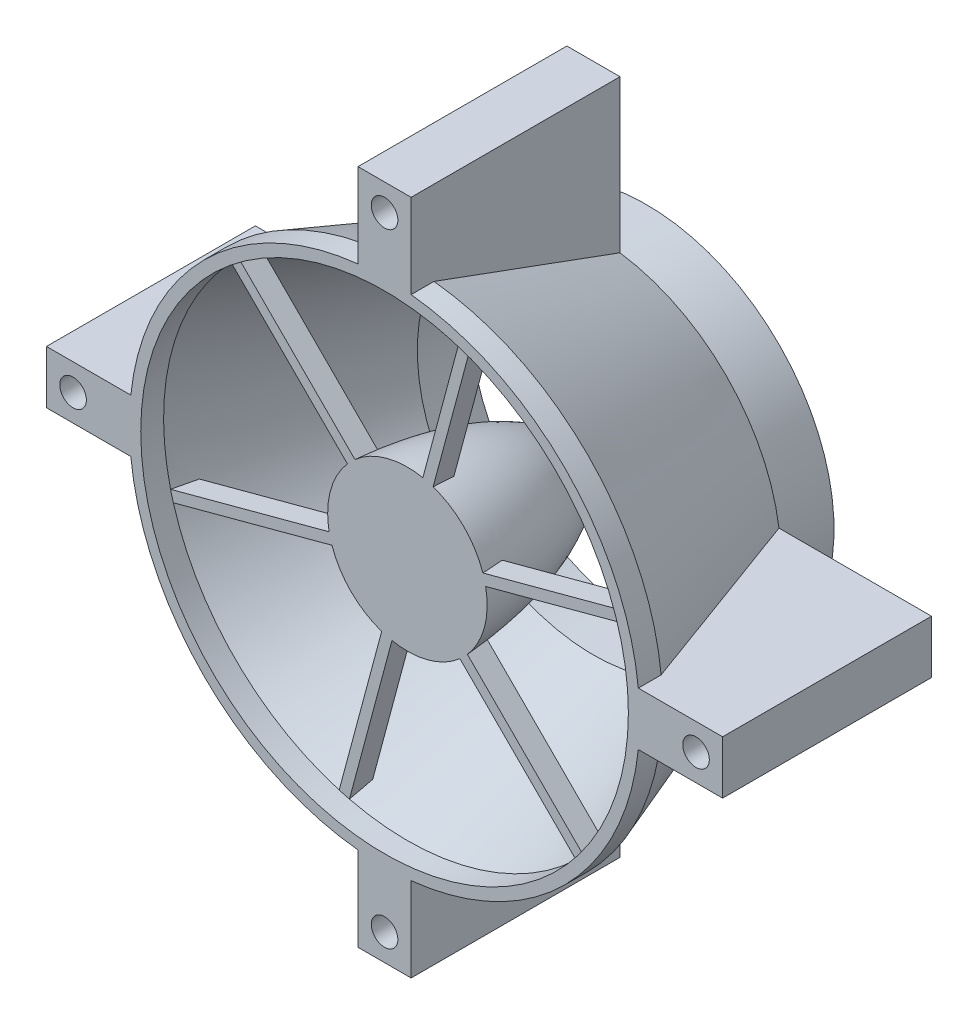
from build123d import *

# Parameters (mm, degrees)
SHELL2_T             = -2
BOSS_EXTRUDE10_REACH = 128.426
SKETCH20_W           = 10
SKETCH20_H           = 35
SKETCH21_R           = 2.5
CUT_EXTRUDE3_DEPTH   = 88.028501079
CIRPATTERN3_COUNT    = 4
SKETCH22_R           = 35.261041801
SKETCH22_R_2         = 33.132686256
BOSS_EXTRUDE11_DEPTH = 10
BOSS_EXTRUDE12_START = -5.388079
SKETCH24_W           = 4
SKETCH24_H           = 2
BOSS_EXTRUDE12_DEPTH = 31.259724
CIRPATTERN4_COUNT    = 6
SKETCH25_R           = 45.871644455
BOSS_EXTRUDE13_DEPTH = 4.3
SKETCH26_R           = 2.5
CUT_EXTRUDE4_DEPTH   = 103.569049913
SKETCH27_R           = 2.5
CUT_EXTRUDE5_DEPTH   = 103.569049913
SKETCH28_R           = 2.5
CUT_EXTRUDE6_DEPTH   = 103.569049913


with BuildPart() as part:
    # Sketch18 → Revolve1 (revolve)
    with BuildSketch(Plane(origin=(0, 0, 0), x_dir=(1, 0, 0), z_dir=(0, 1, 0)), mode=Mode.PRIVATE) as revolve1_sk:
        Polygon((0, 0), (-48, 0), (-35.261041801, 35), (0, 35), align=None)
    revolve(revolve1_sk.sketch.rotate(Axis((0, 0, 0), (0, 0, -1)), 180), axis=Axis((0, 0, 0), (0, 0, -1)))

    # Shell2
    shell2_openings = [part.faces().sort_by_distance(p)[0] for p in [
        (0, 0, -35),
        (0, 0, 0),
    ]]
    offset(amount=SHELL2_T, openings=shell2_openings, kind=Kind.INTERSECTION)

    # Sketch20 → Boss-Extrude10 (add, up to next)
    with BuildSketch(Plane(origin=(0, 63.6, 0), x_dir=(1, 0, 0), z_dir=(0, 1, 0)), mode=Mode.PRIVATE) as boss_extrude10_sk1:
        with Locations((0, 17.5)):
            Rectangle(SKETCH20_W, SKETCH20_H)
    boss_extrude10_tool1 = extrude(boss_extrude10_sk1.sketch, amount=-BOSS_EXTRUDE10_REACH, mode=Mode.PRIVATE) - part.part
    boss_extrude10 = boss_extrude10_tool1.solids().sort_by_distance((0, 63.6, -17.5))[0]
    add(boss_extrude10)

    # Sketch21 → Cut-Extrude3 (cut, through all)
    with BuildSketch(Plane(origin=(0, 0, -35), x_dir=(-1, 0, 0), z_dir=(0, 0, -1))):
        with Locations((0, 58.6)):
            Circle(SKETCH21_R)
    cut_extrude3 = extrude(amount=-CUT_EXTRUDE3_DEPTH, mode=Mode.SUBTRACT)

    # CirPattern3: Boss-Extrude10, Cut-Extrude3 ×4 about axis
    cirpattern3_axis = Axis((0, 0, 0), (0, 0, 1))
    add([boss_extrude10.rotate(cirpattern3_axis, i * 360 / CIRPATTERN3_COUNT) for i in range(1, CIRPATTERN3_COUNT)])
    add([cut_extrude3.rotate(cirpattern3_axis, i * 360 / CIRPATTERN3_COUNT) for i in range(1, CIRPATTERN3_COUNT)], mode=Mode.SUBTRACT)

    # Sketch22 → Boss-Extrude11 (add)
    with BuildSketch(Plane(origin=(0, 0, -35), x_dir=(-1, 0, 0), z_dir=(0, 0, -1))):
        with Locations(Location((0, 0, 0), (0, 0, 171.848007917))):
            Circle(SKETCH22_R)
        with Locations(Location((0, 0, 0), (0, 0, 180))):
            Circle(SKETCH22_R_2, mode=Mode.SUBTRACT)
    extrude(amount=BOSS_EXTRUDE11_DEPTH)



with BuildPart() as body_2:
    # Sketch23 → Revolve2 (revolve)
    with BuildSketch(Plane(origin=(0, 0, 0), x_dir=(1, 0, 0), z_dir=(0, 1, 0))):
        with BuildLine():
            Line((0, 0), (-15, 0))
            add(Edge.make_bspline(
                [(-15, 0), (-14.134412254, 12.425116283), (-11.061625239, 27.366592237), (0, 35)],
                knots=[0, 0, 0, 0, 1, 1, 1, 1], degree=3))
            Line((0, 35), (0, 0))
        make_face()
    revolve(axis=Axis((0, 0, 0), (0, 0, -1)))


with BuildPart() as part_1:
    add(part.part)

    add(body_2.part)  # Boss-Extrude12 merges body 2
    # Sketch24 → Boss-Extrude12 (add)
    with BuildSketch(Plane(origin=(-14.142135624, 14.142135624, 0), x_dir=(0, 0, -1), z_dir=(-0.7071067811865488, 0.7071067811865464, 0)).offset(BOSS_EXTRUDE12_START)):
        with Locations((2, 0)):
            Rectangle(SKETCH24_W, SKETCH24_H)
    boss_extrude12 = extrude(amount=BOSS_EXTRUDE12_DEPTH)

    # CirPattern4: Boss-Extrude12 ×6 about axis
    cirpattern4_axis = Axis((0, 0, 0), (0, 0, 1))
    for i in range(1, CIRPATTERN4_COUNT):
        add(boss_extrude12.rotate(cirpattern4_axis, i * 360 / CIRPATTERN4_COUNT))

    # Sketch25 → Boss-Extrude13 (add)
    with BuildSketch(Plane.XY):
        with BuildLine():
            Line((-47.738873049, 5), (-63.6, 5))
            Line((-63.6, 5), (-63.6, -5))
            Line((-63.6, -5), (-47.738873049, -5))
            ThreePointArc((-47.738873049, -5), (-33.941125497, -33.941125497), (-5, -47.738873049))
            Line((-5, -47.738873049), (-5, -63.6))
            Line((-5, -63.6), (5, -63.6))
            Line((5, -63.6), (5, -47.738873049))
            ThreePointArc((5, -47.738873049), (33.941125497, -33.941125497), (47.738873049, -5))
            Line((47.738873049, -5), (63.6, -5))
            Line((63.6, -5), (63.6, 5))
            Line((63.6, 5), (47.738873049, 5))
            ThreePointArc((47.738873049, 5), (33.941125497, 33.941125497), (5, 47.738873049))
            Line((5, 47.738873049), (5, 63.6))
            Line((5, 63.6), (-5, 63.6))
            Line((-5, 63.6), (-5, 47.738873049))
            ThreePointArc((-5, 47.738873049), (-33.941125497, 33.941125497), (-47.738873049, 5))
        make_face()
        Circle(SKETCH25_R, mode=Mode.SUBTRACT)
    extrude(amount=BOSS_EXTRUDE13_DEPTH)

    # Sketch26 → Cut-Extrude4 (cut, through all)
    with BuildSketch(Plane.XY.offset(4.3)):
        with Locations(Location((-58.6, 0, 0), (0, 0, 270))):
            Circle(SKETCH26_R)
    extrude(amount=-CUT_EXTRUDE4_DEPTH, mode=Mode.SUBTRACT)

    # Sketch27 → Cut-Extrude5 (cut, through all)
    with BuildSketch(Plane.XY.offset(4.3)):
        with Locations(Location((0, 58.6, 0), (0, 0, 180))):
            Circle(SKETCH27_R)
    extrude(amount=-CUT_EXTRUDE5_DEPTH, mode=Mode.SUBTRACT)

    # Sketch28 → Cut-Extrude6 (cut, through all)
    with BuildSketch(Plane.XY.offset(4.3)):
        with Locations((0, -58.6)):
            Circle(SKETCH28_R)
        with Locations(Location((58.6, 0, 0), (0, 0, 90))):
            Circle(SKETCH28_R)
    extrude(amount=-CUT_EXTRUDE6_DEPTH, mode=Mode.SUBTRACT)


solid = part_1.part
